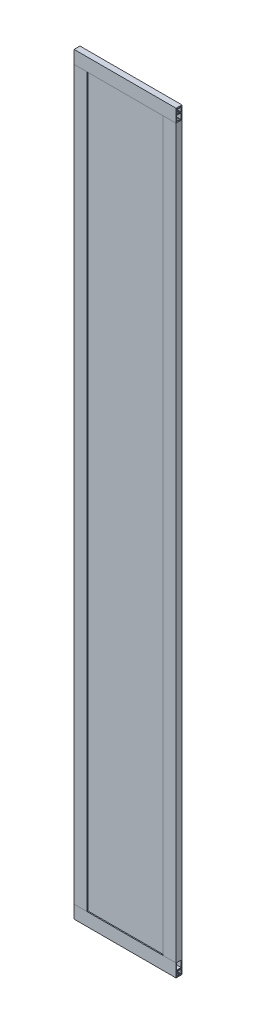
from build123d import *

# Parameters (mm, degrees)
MEMBER_1_DEPTH   = 313.5
MEMBER_1_2_DEPTH = 313.5
MEMBER_1_3_DEPTH = 2319
MEMBER_1_4_DEPTH = 2319
EXTRUDE_START    = -3.1
SKETCH_2_W       = 267.5
SKETCH_2_H       = 2271
EXTRUDE_1_DEPTH  = 10


with BuildPart() as part:
    # Sketch1 → Member 1 (new body)
    with BuildSketch(Plane(origin=(-156.75, 1158.5, 0), x_dir=(0, 0, -1), z_dir=(1, 0, 0))):
        Polygon((7, -38.5), (5.9, -38.5), (5.9, -40), (7, -40), (9, -40), (9, 0), (-9, 0), (-9, -40), (-7, -40), (-5.9, -40), (-5.9, -38.5), (-7, -38.5), (-7, -20), (7, -20), align=None)
        with BuildLine():
            Line((-1.341640786, -18), (1.341640786, -18))
            ThreePointArc((1.341640786, -18), (1.799302724, -16.749903013), (1.272792206, -15.527207794))
            ThreePointArc((1.272792206, -15.527207794), (1.272792206, -14.749390335), (2.050609665, -14.749390335))
            ThreePointArc((2.050609665, -14.749390335), (2.853462499, -16.282552641), (2.640075756, -18))
            Line((2.640075756, -18), (7, -18))
            Line((7, -18), (7, -3))
            Line((7, -3), (2.640075756, -3))
            ThreePointArc((2.640075756, -3), (2.853462499, -4.717447359), (2.050609665, -6.250609665))
            ThreePointArc((2.050609665, -6.250609665), (1.272792206, -6.250609665), (1.272792206, -5.472792206))
            ThreePointArc((1.272792206, -5.472792206), (1.799302724, -4.250096987), (1.341640786, -3))
            Line((1.341640786, -3), (-1.341640786, -3))
            ThreePointArc((-1.341640786, -3), (-1.799302724, -4.250096987), (-1.272792206, -5.472792206))
            ThreePointArc((-1.272792206, -5.472792206), (-1.272792206, -6.250609665), (-2.050609665, -6.250609665))
            ThreePointArc((-2.050609665, -6.250609665), (-2.853462499, -4.717447359), (-2.640075756, -3))
            Line((-2.640075756, -3), (-7, -3))
            Line((-7, -3), (-7, -18))
            Line((-7, -18), (-2.640075756, -18))
            ThreePointArc((-2.640075756, -18), (-2.853462499, -16.282552641), (-2.050609665, -14.749390335))
            ThreePointArc((-2.050609665, -14.749390335), (-1.272792206, -14.749390335), (-1.272792206, -15.527207794))
            ThreePointArc((-1.272792206, -15.527207794), (-1.799302724, -16.749903013), (-1.341640786, -18))
        make_face(mode=Mode.SUBTRACT)
    extrude(amount=MEMBER_1_DEPTH)


with BuildPart() as body_2:
    # Sketch1 on segment 2 (carried to segment 2) → Member 1 2 (new body)
    with BuildSketch(Plane(origin=(-156.75, -1158.5, 0), x_dir=(0, 0, 1), z_dir=(1, 0, 0))):
        Polygon((7, -38.5), (5.9, -38.5), (5.9, -40), (7, -40), (9, -40), (9, 0), (-9, 0), (-9, -40), (-7, -40), (-5.9, -40), (-5.9, -38.5), (-7, -38.5), (-7, -20), (7, -20), align=None)
        with BuildLine():
            Line((-1.341640786, -18), (1.341640786, -18))
            ThreePointArc((1.341640786, -18), (1.799302724, -16.749903013), (1.272792206, -15.527207794))
            ThreePointArc((1.272792206, -15.527207794), (1.272792206, -14.749390335), (2.050609665, -14.749390335))
            ThreePointArc((2.050609665, -14.749390335), (2.853462499, -16.282552641), (2.640075756, -18))
            Line((2.640075756, -18), (7, -18))
            Line((7, -18), (7, -3))
            Line((7, -3), (2.640075756, -3))
            ThreePointArc((2.640075756, -3), (2.853462499, -4.717447359), (2.050609665, -6.250609665))
            ThreePointArc((2.050609665, -6.250609665), (1.272792206, -6.250609665), (1.272792206, -5.472792206))
            ThreePointArc((1.272792206, -5.472792206), (1.799302724, -4.250096987), (1.341640786, -3))
            Line((1.341640786, -3), (-1.341640786, -3))
            ThreePointArc((-1.341640786, -3), (-1.799302724, -4.250096987), (-1.272792206, -5.472792206))
            ThreePointArc((-1.272792206, -5.472792206), (-1.272792206, -6.250609665), (-2.050609665, -6.250609665))
            ThreePointArc((-2.050609665, -6.250609665), (-2.853462499, -4.717447359), (-2.640075756, -3))
            Line((-2.640075756, -3), (-7, -3))
            Line((-7, -3), (-7, -18))
            Line((-7, -18), (-2.640075756, -18))
            ThreePointArc((-2.640075756, -18), (-2.853462499, -16.282552641), (-2.050609665, -14.749390335))
            ThreePointArc((-2.050609665, -14.749390335), (-1.272792206, -14.749390335), (-1.272792206, -15.527207794))
            ThreePointArc((-1.272792206, -15.527207794), (-1.799302724, -16.749903013), (-1.341640786, -18))
        make_face(mode=Mode.SUBTRACT)
    extrude(amount=MEMBER_1_2_DEPTH)


with BuildPart() as body_3:
    # Sketch1 on segment 3 (carried to segment 3) → Member 1 3 (new body)
    with BuildSketch(Plane(origin=(-156.75, 1159.5, 0), x_dir=(0, 0, 1), z_dir=(0, -1, 0))):
        Polygon((7, -38.5), (5.9, -38.5), (5.9, -40), (7, -40), (9, -40), (9, 0), (-9, 0), (-9, -40), (-7, -40), (-5.9, -40), (-5.9, -38.5), (-7, -38.5), (-7, -20), (7, -20), align=None)
        with BuildLine():
            Line((-1.341640786, -18), (1.341640786, -18))
            ThreePointArc((1.341640786, -18), (1.799302724, -16.749903013), (1.272792206, -15.527207794))
            ThreePointArc((1.272792206, -15.527207794), (1.272792206, -14.749390335), (2.050609665, -14.749390335))
            ThreePointArc((2.050609665, -14.749390335), (2.853462499, -16.282552641), (2.640075756, -18))
            Line((2.640075756, -18), (7, -18))
            Line((7, -18), (7, -3))
            Line((7, -3), (2.640075756, -3))
            ThreePointArc((2.640075756, -3), (2.853462499, -4.717447359), (2.050609665, -6.250609665))
            ThreePointArc((2.050609665, -6.250609665), (1.272792206, -6.250609665), (1.272792206, -5.472792206))
            ThreePointArc((1.272792206, -5.472792206), (1.799302724, -4.250096987), (1.341640786, -3))
            Line((1.341640786, -3), (-1.341640786, -3))
            ThreePointArc((-1.341640786, -3), (-1.799302724, -4.250096987), (-1.272792206, -5.472792206))
            ThreePointArc((-1.272792206, -5.472792206), (-1.272792206, -6.250609665), (-2.050609665, -6.250609665))
            ThreePointArc((-2.050609665, -6.250609665), (-2.853462499, -4.717447359), (-2.640075756, -3))
            Line((-2.640075756, -3), (-7, -3))
            Line((-7, -3), (-7, -18))
            Line((-7, -18), (-2.640075756, -18))
            ThreePointArc((-2.640075756, -18), (-2.853462499, -16.282552641), (-2.050609665, -14.749390335))
            ThreePointArc((-2.050609665, -14.749390335), (-1.272792206, -14.749390335), (-1.272792206, -15.527207794))
            ThreePointArc((-1.272792206, -15.527207794), (-1.799302724, -16.749903013), (-1.341640786, -18))
        make_face(mode=Mode.SUBTRACT)
    extrude(amount=MEMBER_1_3_DEPTH)

    # Member 1 3 end butt 1
    split(bisect_by=Plane(origin=(-156.75, 1118.5, 0), x_dir=(1, 0, 0), z_dir=(0, -1, 0)), keep=Keep.TOP)

    # Member 1 3 end butt 2
    split(bisect_by=Plane(origin=(-156.75, -1118.5, 0), x_dir=(-1, 0, 0), z_dir=(0, 1, 0)), keep=Keep.TOP)


with BuildPart() as body_4:
    # Sketch1 on segment 4 (carried to segment 4) → Member 1 4 (new body)
    with BuildSketch(Plane(origin=(156.75, 1159.5, 0), x_dir=(0, 0, -1), z_dir=(0, -1, 0))):
        Polygon((7, -38.5), (5.9, -38.5), (5.9, -40), (7, -40), (9, -40), (9, 0), (-9, 0), (-9, -40), (-7, -40), (-5.9, -40), (-5.9, -38.5), (-7, -38.5), (-7, -20), (7, -20), align=None)
        with BuildLine():
            Line((-1.341640786, -18), (1.341640786, -18))
            ThreePointArc((1.341640786, -18), (1.799302724, -16.749903013), (1.272792206, -15.527207794))
            ThreePointArc((1.272792206, -15.527207794), (1.272792206, -14.749390335), (2.050609665, -14.749390335))
            ThreePointArc((2.050609665, -14.749390335), (2.853462499, -16.282552641), (2.640075756, -18))
            Line((2.640075756, -18), (7, -18))
            Line((7, -18), (7, -3))
            Line((7, -3), (2.640075756, -3))
            ThreePointArc((2.640075756, -3), (2.853462499, -4.717447359), (2.050609665, -6.250609665))
            ThreePointArc((2.050609665, -6.250609665), (1.272792206, -6.250609665), (1.272792206, -5.472792206))
            ThreePointArc((1.272792206, -5.472792206), (1.799302724, -4.250096987), (1.341640786, -3))
            Line((1.341640786, -3), (-1.341640786, -3))
            ThreePointArc((-1.341640786, -3), (-1.799302724, -4.250096987), (-1.272792206, -5.472792206))
            ThreePointArc((-1.272792206, -5.472792206), (-1.272792206, -6.250609665), (-2.050609665, -6.250609665))
            ThreePointArc((-2.050609665, -6.250609665), (-2.853462499, -4.717447359), (-2.640075756, -3))
            Line((-2.640075756, -3), (-7, -3))
            Line((-7, -3), (-7, -18))
            Line((-7, -18), (-2.640075756, -18))
            ThreePointArc((-2.640075756, -18), (-2.853462499, -16.282552641), (-2.050609665, -14.749390335))
            ThreePointArc((-2.050609665, -14.749390335), (-1.272792206, -14.749390335), (-1.272792206, -15.527207794))
            ThreePointArc((-1.272792206, -15.527207794), (-1.799302724, -16.749903013), (-1.341640786, -18))
        make_face(mode=Mode.SUBTRACT)
    extrude(amount=MEMBER_1_4_DEPTH)

    # Member 1 4 end butt 1
    split(bisect_by=Plane(origin=(156.75, 1118.5, 0), x_dir=(1, 0, 0), z_dir=(0, -1, 0)), keep=Keep.TOP)

    # Member 1 4 end butt 2
    split(bisect_by=Plane(origin=(156.75, -1118.5, 0), x_dir=(-1, 0, 0), z_dir=(0, 1, 0)), keep=Keep.TOP)


with BuildPart() as body_5:
    # 草图2 → 凸台-拉伸1 (new body)
    with BuildSketch(Plane.XY.offset(9).offset(EXTRUDE_START)):
        Rectangle(SKETCH_2_W, SKETCH_2_H)
    extrude(amount=-EXTRUDE_1_DEPTH)


solid = Compound([part.part, body_2.part, body_3.part, body_4.part, body_5.part])
